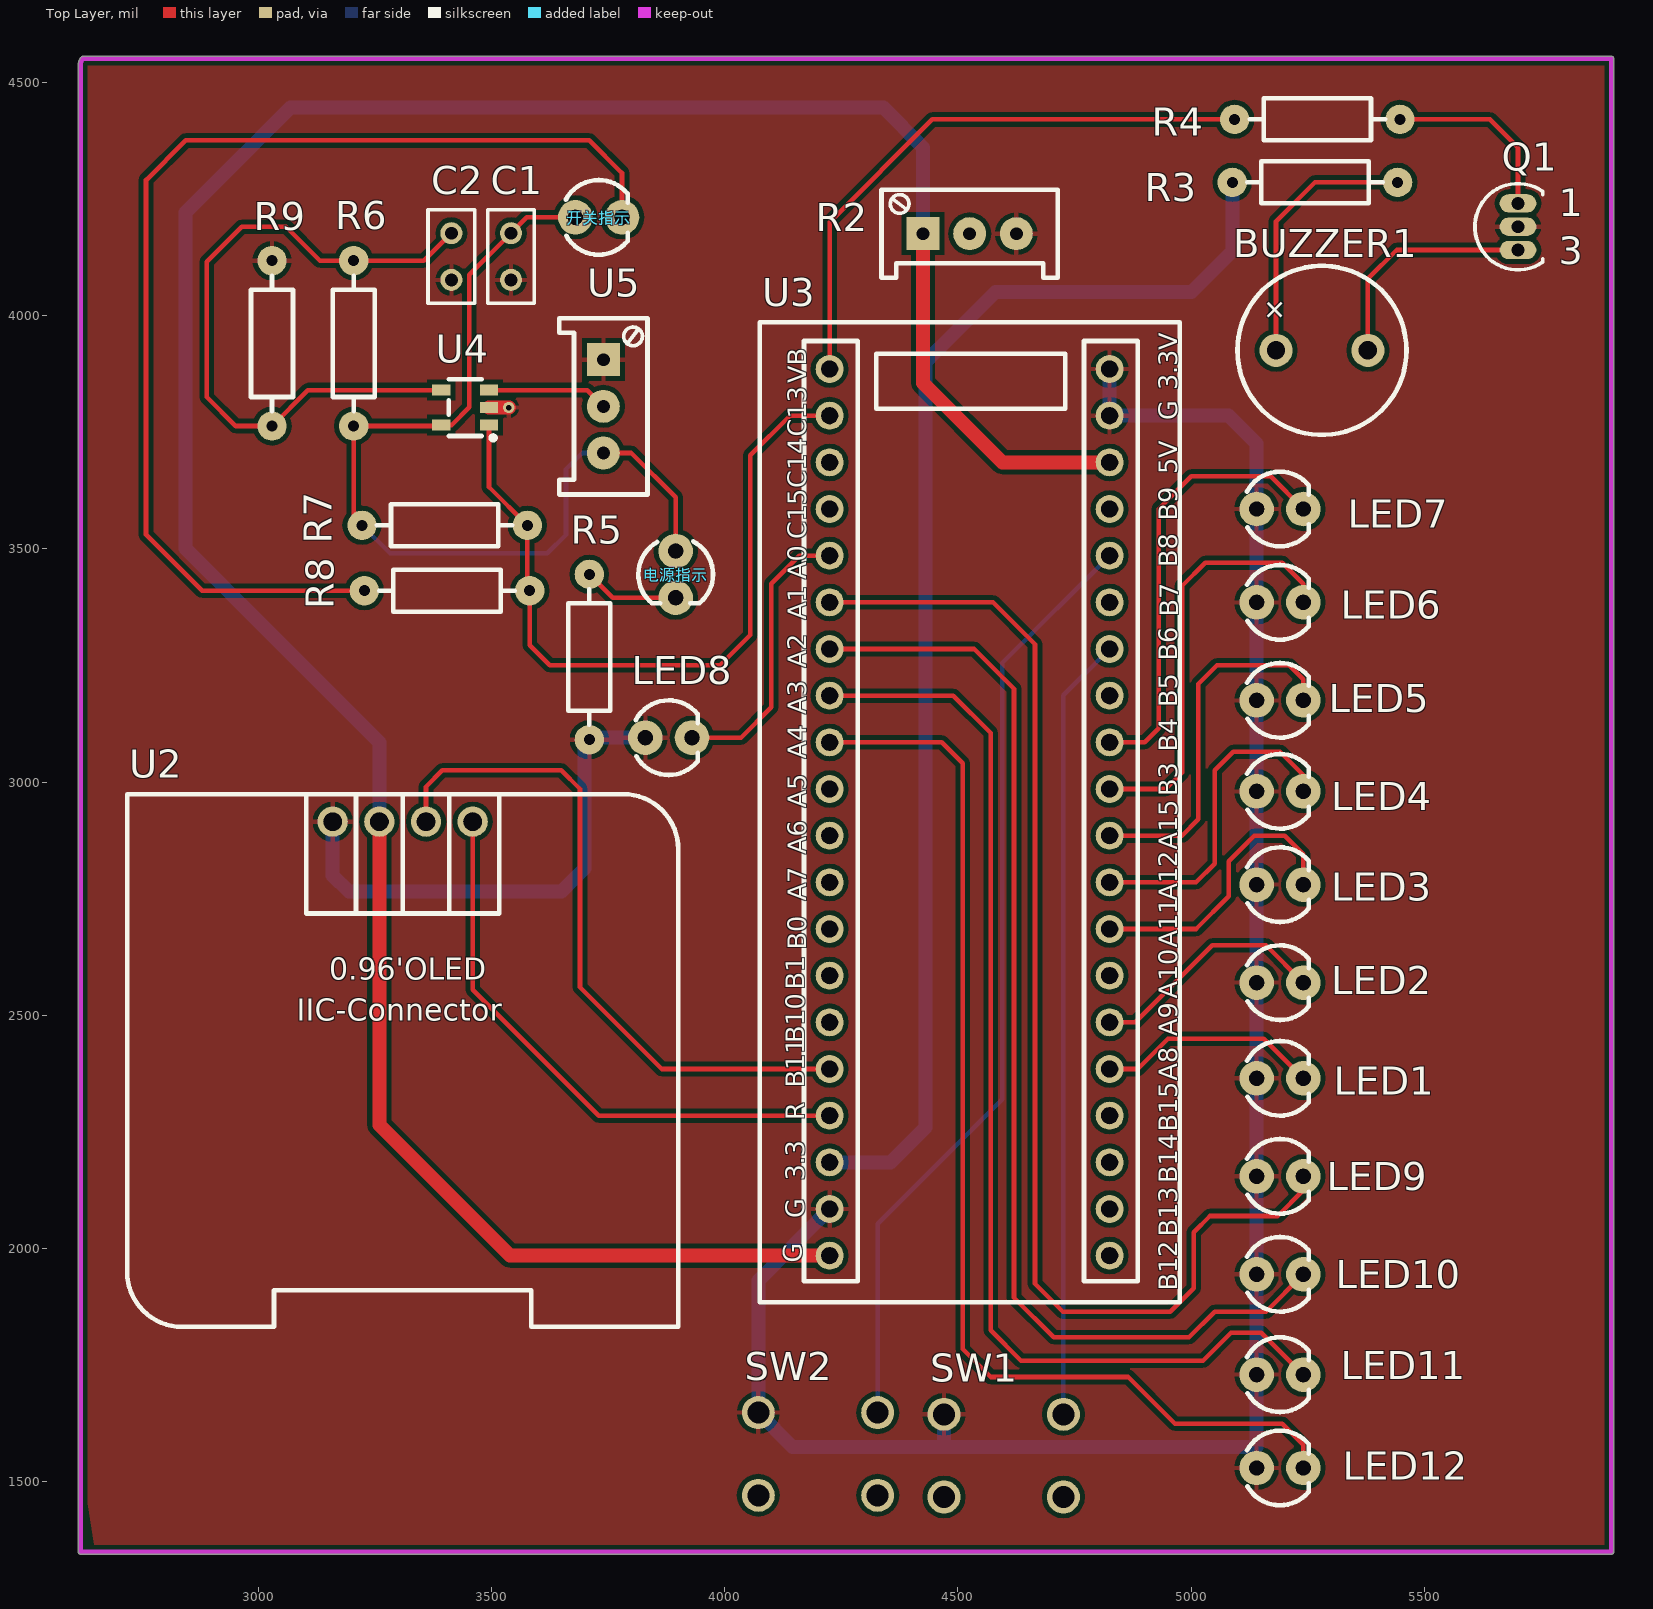
[diagram p0: Top Layer view]
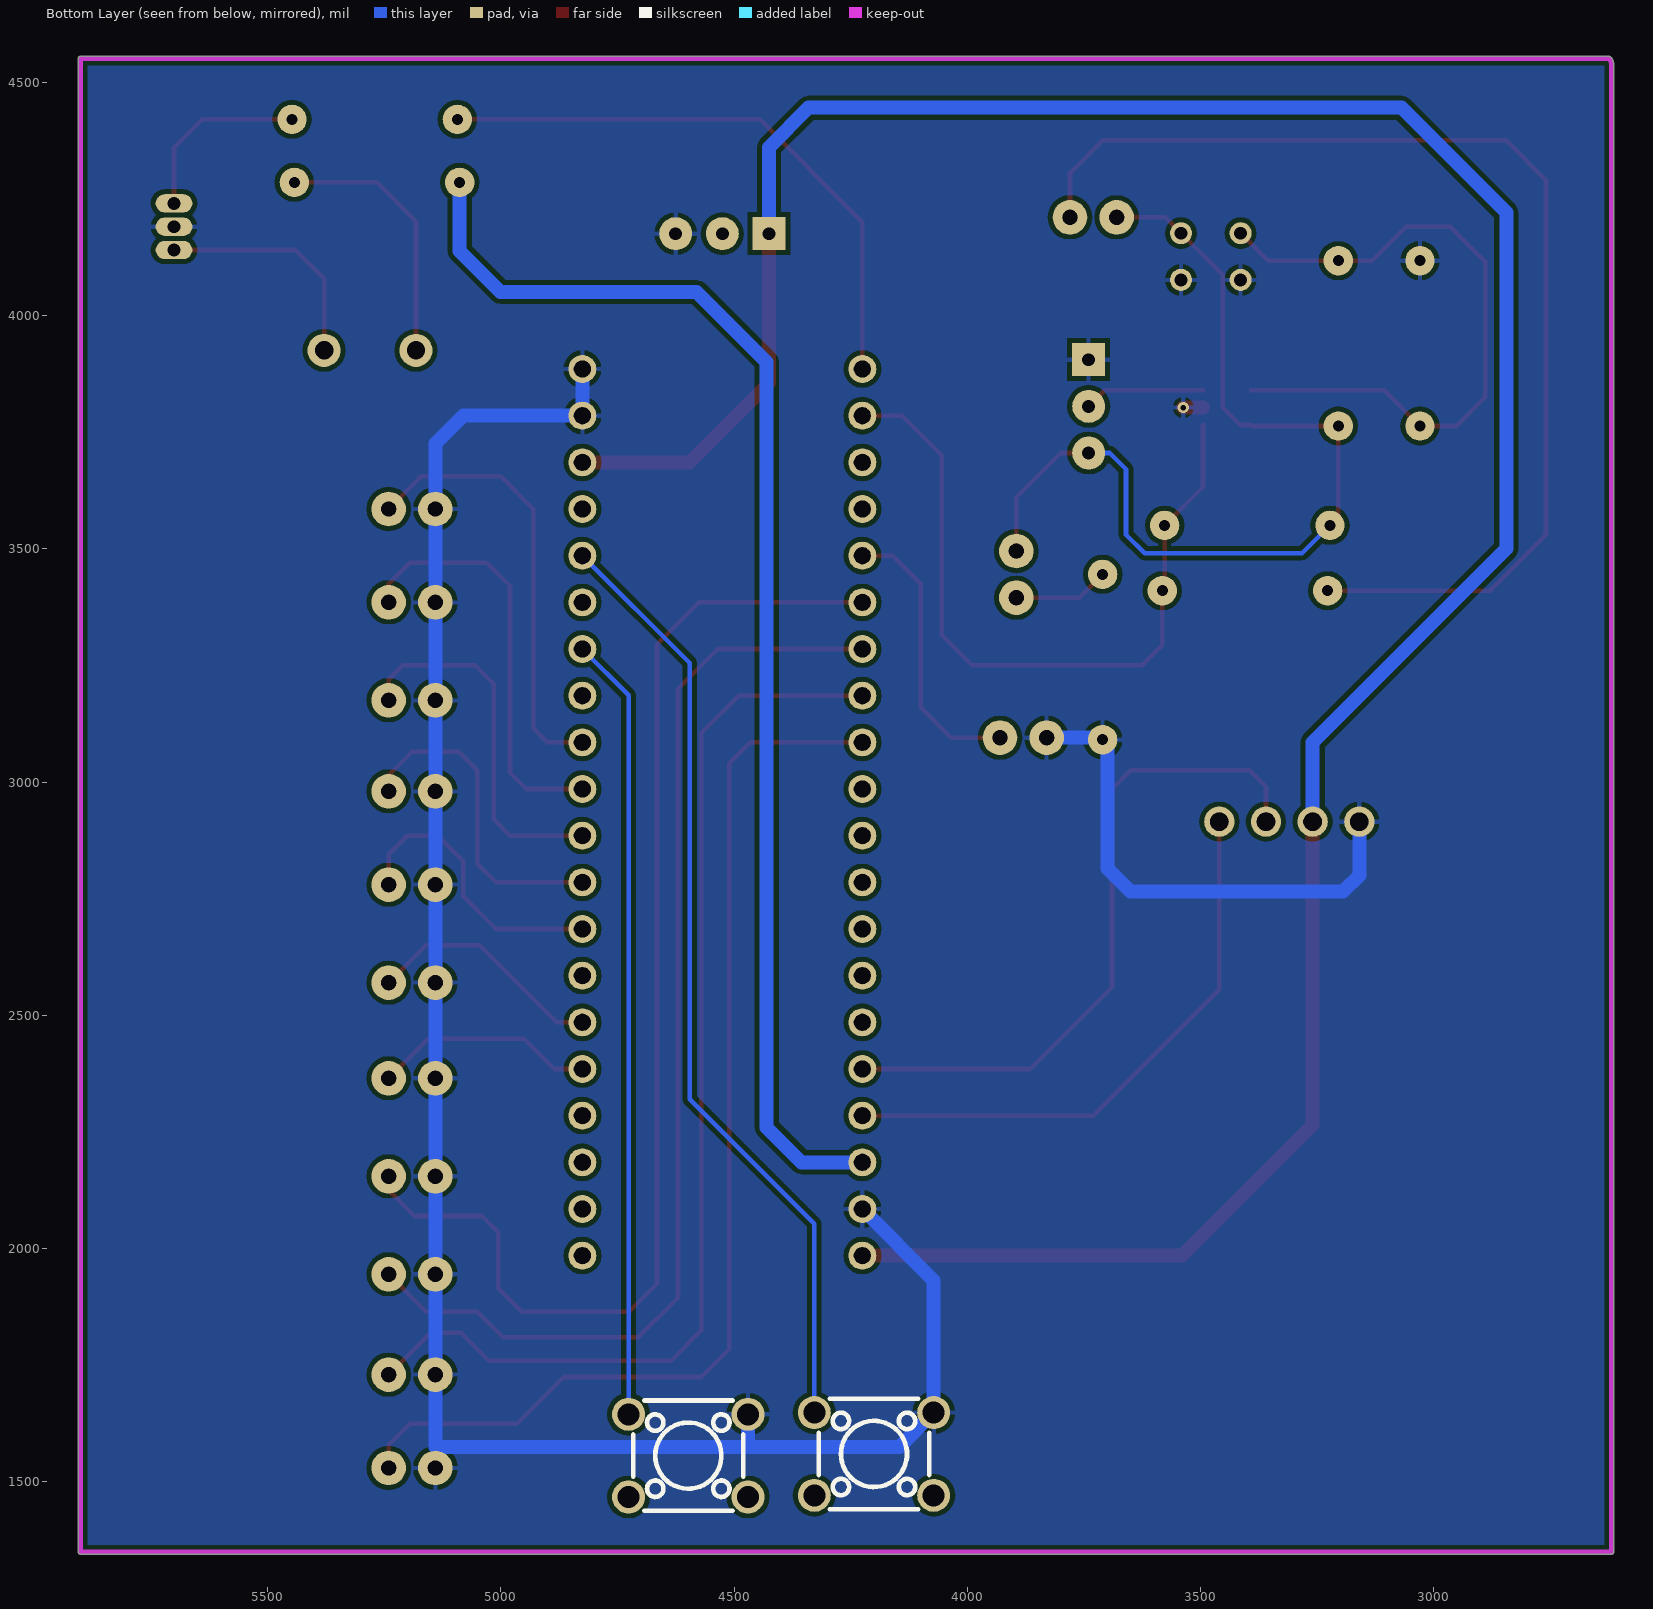
[diagram p1: Bottom Layer view, seen from below]
# Altium PCB MISC80522.PcbDoc
Units mil, origin at the board's own origin, x right, y up, seen from the top; angles counter-clockwise.
Board outline 3290.03 x 3210.03 mil, 2 copper layers (Top Layer, Bottom Layer); 32 components, 30 nets, 114 pads, 1 vias.

## Layer stack, top to bottom (the 12.6 mil dielectric is the usual default, probably not edited)
Top Solder: solder mask 0.4, Solder Resist, Dk 3.5
Top Layer: signal copper 1.4
Dielectric 1: dielectric 12.6, FR-4, Dk 4.8
Bottom Layer: signal copper 1.4
Bottom Solder: solder mask 0.4, Solder Resist, Dk 3.5

## Board outline
2614.99,1350 ccw(c2620,1350) 2620,1344.98 5900,1344.98 ccw(c5900,1350) 5905.02,1350 5905.02,4550 ccw(c5900,4550) 5900,4555.02 2625,4555.02 ccw(c2625,4550) 2621.45,4553.55 ccw(c2637.07,4537.93) 2614.99,4537.93

## Design rules (kind name [scope] priority, off if disabled: settings)
Clearance [All] p1: gap=10
MinimumSolderMaskSliver [All] p1: minsoldermaskwidth=0
PolygonConnect [All] p1: connectstyle=Relief reliefconductorwidth=10 reliefentries=4 polygonreliefangle="90 Angle" airgapwidth=10
RoutingVias [All] p1: holewidth=28 width=50 viastyle="Through Hole" minholewidth=28 minwidth=50 maxholewidth=28 maxwidth=50
SilkToSilkClearance [All] p1: silktosilkclearance=0
SilkToSolderMaskClearance [IsPad] p1: minsilkscreentomaskgap=0 clearancetoexposedcopper=TRUE
SolderMaskExpansion [All] p1: expansion=4
Width [All] p1: maxlimit=30 minlimit=10 preferedwidth=10
27 further rules are at their usual default settings.

## Components (designator, comment, footprint, x,y, rotation, side; value= is the part's Value field where it differs from the comment)
BUZZER1 "2.4kHz" BUZZER 5280,3925 r0 top
C1 "104" RAD-0.1 3542.13,4126.06 r90 top
C2 "100nF" RAD-0.1 3414.25,4126.06 r90 top
LED1 "LTST-C190KSKT" LED3MM 5190,2365 r0 top
LED2 "LTST-C190KSKT" LED3MM 5190,2570 r0 top
LED3 "LTST-C190KSKT" LED3MM 5190,2780 r0 top
LED4 "LTST-C190KSKT" LED3MM 5190,2980 r0 top
LED5 "LTST-C190KSKT" LED3MM 5190,3175 r0 top
LED6 "LTST-C190KSKT" LED3MM 5190,3385 r0 top
LED7 "LTST-C190KSKT" LED3MM 5190,3585 r0 top
LED8 "LTST-C190KSKT" LED3MM 3880,3095 r0 top
LED9 "LTST-C190KSKT" LED3MM 5190,2155 r0 top
LED10 "LTST-C190KSKT" LED3MM 5190,1945 r0 top
LED11 "LTST-C190KSKT" LED3MM 5190,1730 r0 top
LED12 "LTST-C190KSKT" LED3MM 5190,1530 r0 top
Q1 "SS8050" TO-92 5700,4190 r0 top
R2 "500kΩ" 3296W 4525,4175 r0 top
R3 "100" "RS 1/4W" 5265,4285 r180 top
R4 "1kΩ" "RS 1/4W" 5270,4420 r0 top
R5 "1000Ω" "RS 1/4W" 3710,3267.83 r90 top
R6 "10000" "RS 1/4W" 3205,3940 r270 top
R7 "10000" "RS 1/4W" 3400,3550 r180 top
R8 "1000Ω" "RS 1/4W" 3405,3410 r180 top
R9 "GL5506(4-7K)" "RS 1/4W" 3030,3940 r90 top
SW1 "TS-1101-C-W" 四脚轻触开关 4597.95,1556.42 r0 top
SW2 "TS-1101-C-W" 四脚轻触开关 4200,1560 r0 top
U2 "HS96L03W2C03" 0.96OLED_4P 3310.05,2403.2 r0 top
U3 "LCKFB-DKX-STM32F103C8T6" STM32核心板 5726.5,3159 r0 top
U4 "TLV3201AIDBVR" SOT-23-5_L3.0-W1.7-P0.95-LS2.8-BR 3443.82,3800.41 r0 top
U5 "res2k3*3*1MM" 3296W 3740,3805 r270 top
开关指示 "KT-0805G" LED3MM 3730,4210 r0 top
电源指示 "KT-0805G" LED3MM 3895,3445 r270 top

## Footprints (in the part's own frame and the unit in brackets; to place one, negate y for a bottom-side part, rotate by r counter-clockwise, add the part's x,y. Pads: shape width x height; smd on the part's side, far side on the other; paste and mask are expansions set on the pad)
0.96OLED_4P [mm]
  round 1.65 hole 1 slot 1.005 at 0 deg paste+0 mask+0.051: 1(-3.811,12.997) 2(-1.271,13) 3(1.269,13) 4(3.809,13)
  silkscreen extent -15,-14.5 15,14.5
3296W [mm] "Precise Multi-Winding Adjustable Resistor"
  rect 1.8x1.8 hole 0.7: 1(-2.54,0)
  round 1.8 hole 0.7: 2(0,0) 3(2.54,0)
  silkscreen extent -4.8,-2.4 4.8,2.4, body extent -4.75,-2.4 4.75,2.4, height 11.52
BUZZER [mm]
  round 1.8 hole 1 paste+0 mask+0.051: 1(-2.5,0) 2(2.5,0)
  silkscreen extent -4.6,-4.6 4.6,4.6
LED3MM [mil]
  round 74 hole 32 slot 32.2 at 0 deg paste+0 mask+2: 1(-50,0) 2(50,0)
  silkscreen extent -71,-80 62,80
RAD-0.1 [mm] "Radial Cap, Thru-Hole; 2 Leads; 0.1 in Pin Spacing"
  round 1.2 hole 0.7: 1(-1.27,0) 2(1.27,0)
  silkscreen extent -2.54,-1.27 2.54,1.27
"RS 1/4W" [mm] "直插色环电阻，脚距9mm，直径2.3mm"
  round 1.6 hole 0.6: 1(-4.5,0) 2(4.5,0)
  silkscreen extent -3.68,-1.14 3.68,1.14, body extent -4.72,-1.16 4.73,1.16, height 2.32
SOT-23-5_L3.0-W1.7-P0.95-LS2.8-BR [mm]
  rect 1x0.6 smd paste+0 mask+0.051: 1(1.3,-0.899) 2(1.3,0.051) 3(1.3,1) 4(-1.3,1) 5(-1.3,-0.899)
  silkscreen extent -0.9,-1.73 1.65,1.6
STM32核心板 [mil]
  round 60 hole 36 slot 36.2 at 0 deg paste+0 mask+2: 1(-1501.5,726) 2(-1501.5,626) 3(-1501.5,526) 4(-1501.5,426) 5(-1501.5,326) 6(-1501.5,226) 7(-1501.5,126) 8(-1501.5,26) 9(-1501.5,-74) 10(-1501.5,-174) 11(-1501.5,-274) 12(-1501.5,-374) 13(-1501.5,-474) 14(-1501.5,-574) 15(-1501.5,-674) 16(-1501.5,-774) 17(-1501.5,-874) 18(-1501.5,-974) 19(-1501.5,-1074) 20(-1501.5,-1174) 21(-901.5,-1174) 22(-901.5,-1074) 23(-901.5,-974) 24(-901.5,-874) 25(-901.5,-774) 26(-901.5,-674) 27(-901.5,-574) 28(-901.5,-474) 29(-901.5,-374) 30(-901.5,-274) 31(-901.5,-174) 32(-901.5,-74) 33(-901.5,26) 34(-901.5,126) 35(-901.5,226) 36(-901.5,326) 37(-901.5,426) 38(-901.5,526) 39(-901.5,626) 40(-901.5,726)
  silkscreen extent -1652,-1274 -752,826
TO-92 [mm] "TO, Flat Index; 3 In-Line, Axial Leads; Body Dia. 4.6mm; Leads 0.41 x 0.39 mm (max)"
  oval 2x1 hole 0.7: 1(0,1.27) 2(0,0) 3(0,-1.27)
  silkscreen extent -2.34,-2.34 1.35,2.34
四脚轻触开关 [mm]
  round 1.8 hole 1.2 paste+0 mask+0.102: 1(3.25,2.25) 2(-3.25,2.25) 3(3.25,-2.25) 4(-3.25,-2.25)

## Part data
BUZZER1: library part TMB12A05_C96093
C1 C2: library part 0603F104Z500CT_C83060
Q1: library part SS8050_C7420370
R2: library part 3362W-1-504LF
R3: library part RE1206F1R050
R4: library part FCR0603F1K
R5 R6 R7 R8: library part HVLR2505F1G00K9
R9: library part GL5506（4-7K）

## Via types
v1: diameter 24, hole 12, Top Layer to Bottom Layer, 1 vias

## Nets (pads, with @x,y where several pads share a name; then routed paths per layer and width w, separated by ;. In a path a pad name is that pad's centre, name@x,y a point inside that pad or via, vN(x,y) a via of type N, cw(c..) or ccw(c..) an arc to the next point about the centre after c; other vN are vias at no path point)
+3.3V: R2.1 U2.2 U3.20 U3.38 | length 5891.7
  Top Layer w30: U2.2 3260,2265 3540,1985 U3.20 ; R2.1 4425,3855 4595,3685 U3.38
  Bottom Layer w30: U2.2 3260,3085 2845,3500 2845,4220 3070,4445 4340,4445 4425,4360 R2.1
+5V: R3.2 U3.18 | length 2779.6
  Bottom Layer w30: U3.18 4355,2185 4430,2260 4430,3900 4580,4050 5000,4050 5087.83,4137.83 R3.2
A0: LED1.2 U3.25 | length 477.1
  Top Layer w10: U3.25 4885,2385 4950,2450 5155,2450 LED1.2
A1: LED2.2 U3.26 | length 516.5
  Top Layer w10: U3.26 4880,2485 5045,2650 5160,2650 LED2.2
A2: U3.27
A3: LED3.2 U3.28 | length 623.3
  Top Layer w10: U3.28 5010,2685 5080,2755 5080,2830 5135,2885 5200,2885 5240,2845 LED3.2
A4: LED4.2 U3.29 | length 703.8
  Top Layer w10: U3.29 5010,2785 5050,2825 5050,3025 5090,3065 5190,3065 5240,3015 LED4.2
A5: LED5.2 U3.30 | length 793.5
  Top Layer w10: U3.30 4980,2885 5015,2920 5015,3210 5055,3250 5210,3250 5240,3220 LED5.2
A6: LED6.2 U3.31 | length 908.8
  Top Layer w10: U3.31 4945,2985 4980,3020 4980,3420 5030,3470 5195,3470 5240,3425 LED6.2
A7: LED7.2 U3.32 | length 955.4
  Top Layer w10: U3.32 4900,3085 4930,3115 4930,3585 5000,3655 5170,3655 LED7.2
A8: LED8.2 U3.5 | length 611.8
  Top Layer w10: LED8.2 4035,3095 4100,3160 4100,3425 4160,3485 U3.5
A9: LED9.2 U3.6 | length 2655.1
  Top Layer w10: U3.6 4575,3385 4665,3295 4665,1925 4725,1865 4955,1865 5005,1915 5005,2035 5040,2070 5185,2070 5240,2125 LED9.2
A10: LED10.2 U3.7 | length 2446.3
  Top Layer w10: U3.7 4535,3285 4620,3200 4620,1895 4705,1810 4995,1810 5050,1865 5160,1865 LED10.2
A11: LED11.2 U3.8 | length 2417.2
  Top Layer w10: U3.8 4490,3185 4570,3105 4570,1825 4635,1760 5025,1760 5085,1820 5150,1820 LED11.2
A12: LED12.2 U3.9 | length 2423.6
  Top Layer w10: U3.9 4465,3085 4510,3040 4510,1785 4570,1725 4865,1725 4965,1625 5195,1625 5240,1580 LED12.2
B1: SW1.1 U3.34 | length 1681
  Bottom Layer w10: SW1.1 4725.91,3185.91 U3.34
B8: U2.3 U3.16 | length 1468.6
  Top Layer w10: U2.3 3360,2990 3395,3025 3650,3025 3690,2985 3690,2560 3865,2385 U3.16
B9: U2.4 U3.17 | length 1236.8
  Top Layer w10: U2.4 3460,2555 3730,2285 U3.17
B11: SW2.1 U3.36 | length 2042.3
  Bottom Layer w10: SW2.1 4327.95,2052.95 4595,2320 4595,3255 U3.36
B12: R4.1 U3.1 | length 1274
  Top Layer w10: U3.1 4225,4200 4445,4420 R4.1
B13: R7.1 R8.1 U3.2 U4.1 | length 1616
  Top Layer w10: U4.1 3495,3632.17 R7.1 3577.17,3415 R8.1 3582.17,3292.83 3625,3250 3990,3250 4055,3315 4055,3700 4140,3785 U3.2
GND: C1.1 C2.1 LED1.1 LED2.1 LED3.1 LED4.1 LED5.1 LED6.1 LED7.1 LED8.1 LED9.1 LED10.1 LED11.1 LED12.1 Q1.2 R2.3 R5.1 R9.2 SW1.2 SW2.2 U2.1 U3.19 U3.39 U3.40 U4.2 U5.1 | length 5394.2
  Top Layer w30: U4.2 v1(3537.4,3802.4)
  Bottom Layer w30: U2.1 3160,2800 3195,2765 3650,2765 3700,2815 3700,3080.67 R5.1 3714.33,3095 LED8.1 ; U3.19 4072.05,1932.05 SW2.2 4145.63,1575 4465,1575 ; SW1.2 4470,1580 4465,1575 ; U3.40 U3.39 5080,3785 5140,3725 LED7.1 LED6.1 LED5.1 LED4.1 LED3.1 LED2.1 LED1.1 LED9.1 LED10.1 LED11.1 5140,1575 4465,1575
NetBUZZER1_1: BUZZER1.1 R3.1 | length 571.7
  Top Layer w10: BUZZER1.1 5181.57,4201.57 5265,4285 R3.1
NetBUZZER1_2: BUZZER1.2 Q1.3 | length 500.5
  Top Layer w10: BUZZER1.2 5378.42,4078.42 5440,4140 Q1.3
NetC1_2: C1.2 R6.2 R7.2 U4.5 U5.3 开关指示.1 电源指示.1 | length 2069.2
  Top Layer w10: R7.2 3205,3567.83 R6.2 3390.46,3762.83 U4.5 3415,3765 3452.87,3802.87 3452.87,4086.81 C1.2 3576.06,4210 开关指示.1 ; U5.3 3800,3705 3895,3610 电源指示.1
  Bottom Layer w10: R7.2 3282.83,3490 3620,3490 3660,3530 3660,3670 3695,3705 U5.3
NetC2_2: C2.2 R6.1 R9.1 U4.4 | length 1460.2
  Top Layer w10: U4.4 3106.97,3839.8 R9.1 2952.17,3762.83 2890,3825 2890,4115 2965,4190 3060,4190 3132.83,4117.17 R6.1 3355.35,4117.17 C2.2
NetQ1_1: Q1.1 R4.2 | length 397.7
  Top Layer w10: R4.2 5640,4420 5700,4360 Q1.1
NetR5_2: R5.2 电源指示.2 | length 205.7
  Top Layer w10: R5.2 3760,3395 电源指示.2
NetR8_2: R8.2 开关指示.2 | length 2456.7
  Top Layer w10: R8.2 2880,3410 2760,3530 2760,4290 2845,4375 3710,4375 3780,4305 开关指示.2
NetU4_3: U4.3 U5.2 | length 259.4
  Top Layer w10: U4.3 3705.2,3839.8 U5.2
pads on no net: R2.2 SW1.3 SW1.4 SW2.3 SW2.4 U3.3 U3.4 U3.10 U3.11 U3.12 U3.13 U3.14 U3.15 U3.21 U3.22 U3.23 U3.24 U3.33 U3.35 U3.37

## Polygon pours and split planes (outlines as drawn)
GND on Top Layer "D" (solid, remove dead copper, pour order 0): 2060,5110 2080,5090 6230,5090 6230,1110 6275,1065 6190,980 2710,980
GND on Bottom Layer "D" (solid, remove dead copper, pour order 2): 1960,4745 6315,4745 6495,4925 6000,4430 6000,760 2090,760 1805,1045

## Keep-outs
Keep-Out Layer:
  lines w10: 2620,3860 2620,4537.93 cw(c2637.07,4537.93) 2625,4550 5900,4550 5900,1800 5900,1350 5705,1350 3090,1350 2620,1350 2620,3905